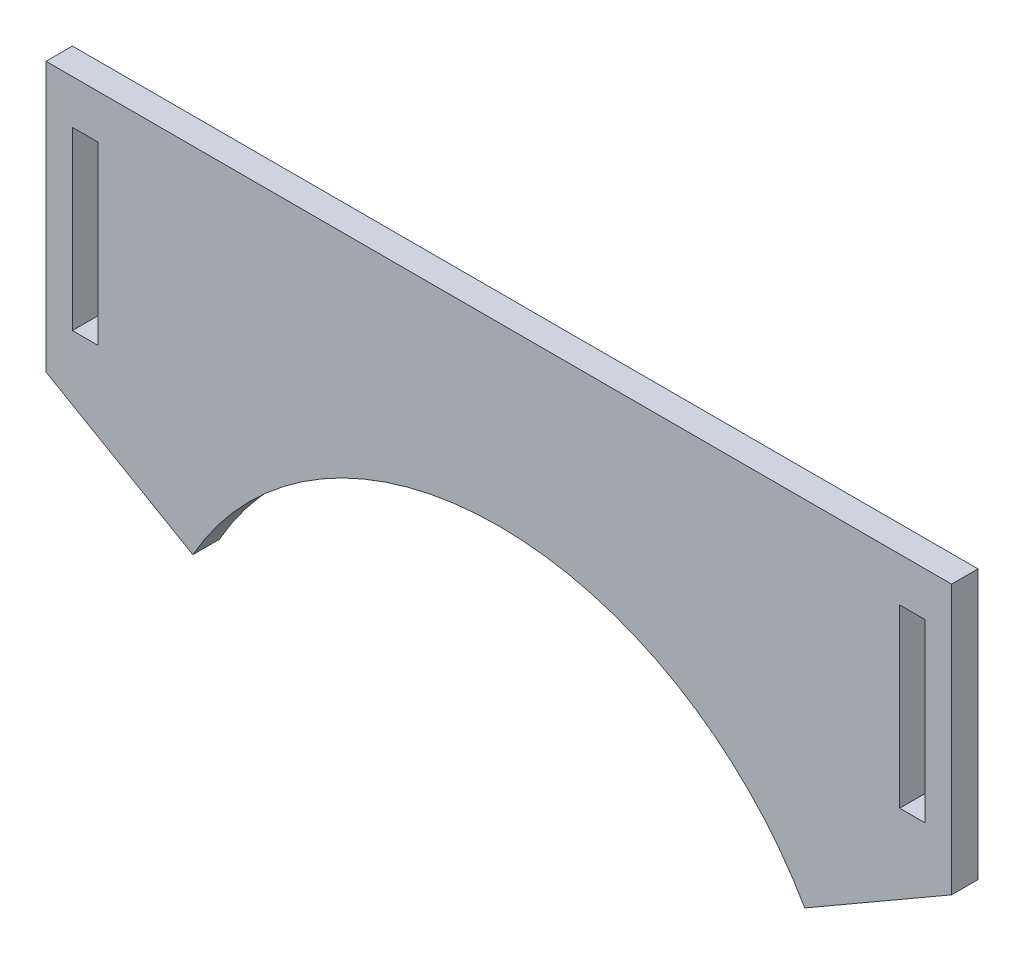
from build123d import *

# Parameters (mm, degrees)
SKETCH1_W           = 2.9
SKETCH1_H           = 20
BOSS_EXTRUDE1_DEPTH = 3
CUT_EXTRUDE1_DEPTH  = 113.383299562


with BuildPart() as part:
    # Sketch1 → Boss-Extrude1 (new body)
    with BuildSketch(Plane.XY):
        with BuildLine():
            Line((0, 0), (104.9, 0))
            Line((104.9, 0), (104.9, -30))
            Line((104.9, -30), (87.212489335, -40.211889044))
            ThreePointArc((87.212489335, -40.211889044), (52.45, -20), (17.687510665, -40.211889044))
            Line((17.687510665, -40.211889044), (0, -30))
            Line((0, -30), (0, 0))
        make_face()
        with Locations((99.45, -15)):
            Rectangle(SKETCH1_W, SKETCH1_H, mode=Mode.SUBTRACT)
        with Locations((5.45, -15)):
            Rectangle(SKETCH1_W, SKETCH1_H, mode=Mode.SUBTRACT)
    extrude(amount=BOSS_EXTRUDE1_DEPTH)

    # Sketch2 → Cut-Extrude1 (cut, through all)
    with BuildSketch(Plane.XY.offset(3)):
        Polygon((1, 0), (1, -30.577350269), (0, -30), (0, 0), align=None)
        Polygon((103.9, 0), (103.9, -30.577350269), (104.9, -30), (104.9, 0), align=None)
    extrude(amount=-CUT_EXTRUDE1_DEPTH, mode=Mode.SUBTRACT)


solid = part.part
